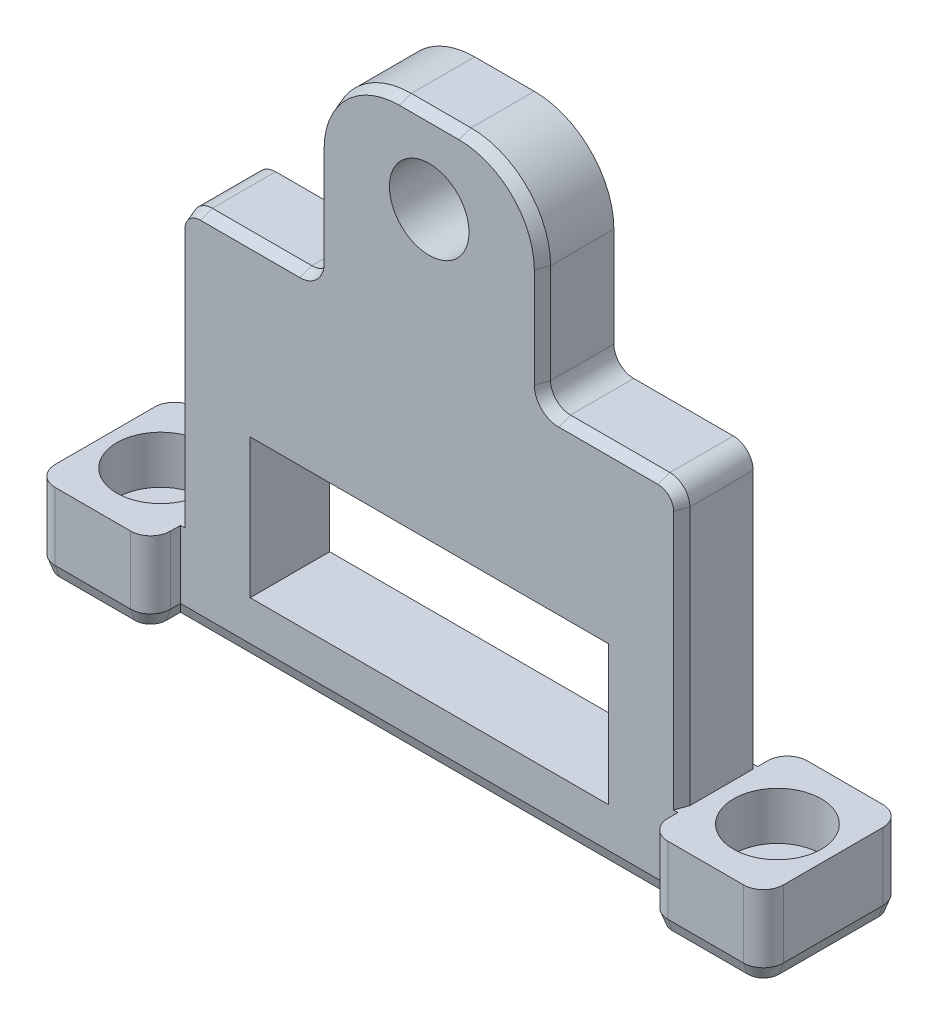
from build123d import *
from OCP.BRepFilletAPI import BRepFilletAPI_MakeChamfer

# Parameters (mm, degrees)
SKETCH1_W           = 12.5
SKETCH1_H           = 14
BOSS_EXTRUDE1_DEPTH = 2
SKETCH2_R           = 1
SKETCH2_W           = 9
SKETCH2_H           = 3.5
SKETCH2_W_2         = 3.5
SKETCH2_H_2         = 5
CUT_EXTRUDE1_DEPTH  = 3
FILLET1_R           = 2
SKETCH4_W           = 2.9
SKETCH4_H           = 3.5
BOSS_EXTRUDE2_DEPTH = 2
SKETCH5_R           = 1.1
CUT_EXTRUDE3_DEPTH  = 1.2
FILLET2_R           = 0.5
FILLET3_R           = 0.5
CHAMFER1_SIZE       = 0.3
CHAMFER1_SIZE2      = 0.10919107


with BuildPart() as part:
    # Sketch1 → Boss-Extrude1 (new body)
    with BuildSketch(Plane.XY):
        Rectangle(SKETCH1_W, SKETCH1_H)
    extrude(amount=BOSS_EXTRUDE1_DEPTH)

    # Sketch2 → Cut-Extrude1 (cut)
    with BuildSketch(Plane.XY.offset(2)):
        with Locations((0, 5)):
            Circle(SKETCH2_R)
        with Locations((0, -3.95)):
            Rectangle(SKETCH2_W, SKETCH2_H)
        with Locations((-4.5, 4.5)):
            Rectangle(SKETCH2_W_2, SKETCH2_H_2)
        with Locations((4.5, 4.5)):
            Rectangle(SKETCH2_W_2, SKETCH2_H_2)
    extrude(amount=-CUT_EXTRUDE1_DEPTH, mode=Mode.SUBTRACT)

    # Fillet1
    fillet1_edges = [part.edges().sort_by_distance(p)[0] for p in [
        (-2.75, 7, 1),
        (2.75, 7, 1),
    ]]
    fillet(fillet1_edges, radius=FILLET1_R)

    # Sketch4 → Boss-Extrude2 (add)
    with BuildSketch(Plane.XZ.offset(7)):
        with Locations((-7.7, 1)):
            Rectangle(SKETCH4_W, SKETCH4_H)
        with Locations((7.7, 1)):
            Rectangle(SKETCH4_W, SKETCH4_H)
    extrude(amount=-BOSS_EXTRUDE2_DEPTH)

    # Sketch5 → Cut-Extrude3 (cut)
    with BuildSketch(Plane(origin=(0, -5, 0), x_dir=(1, 0, 0), z_dir=(0, 1, 0))):
        with Locations(Location((-7.75, -1, 0), (0, 0, 270))):
            Circle(SKETCH5_R)
        with Locations(Location((7.75, -1, 0), (0, 0, 270))):
            Circle(SKETCH5_R)
    extrude(amount=-CUT_EXTRUDE3_DEPTH, mode=Mode.SUBTRACT)

    # Fillet2
    fillet2_edges = [part.edges().sort_by_distance(p)[0] for p in [
        (6.25, -6, -0.75),
        (6.25, -6, 2.75),
        (9.15, -6, 2.75),
        (9.15, -6, -0.75),
        (-6.25, 2, 1),
        (6.25, 2, 1),
        (-6.25, -6, 2.75),
        (-6.25, -6, -0.75),
        (-9.15, -6, -0.75),
        (-9.15, -6, 2.75),
    ]]
    fillet(fillet2_edges, radius=FILLET2_R)

    # Fillet3
    fillet3_edges = [part.edges().sort_by_distance(p)[0] for p in [
        (-2.75, 2, 1),
        (2.75, 2, 1),
    ]]
    fillet(fillet3_edges, radius=FILLET3_R)

    # Chamfer1: one chamfer whose edges measure the first distance from different faces: ONE call of the kernel's chamfer builder (chamfer() names one face for all edges)
    chamfer1_edges_1 = [part.edges().sort_by_distance(p)[0] for p in [
        (-9.003553391, -7, -0.603553391),
    ]]
    chamfer1_side_1 = [part.faces().sort_by_distance(p)[0] for p in [
        (-9.003553391, -6, -0.603553391),
    ]]
    chamfer1_edges_2 = [part.edges().sort_by_distance(p)[0] for p in [
        (-9.15, -7, 1),
    ]]
    chamfer1_side_2 = [part.faces().sort_by_distance(p)[0] for p in [
        (-9.15, -6, 1),
    ]]
    chamfer1_edges_3 = [part.edges().sort_by_distance(p)[0] for p in [
        (-9.003553391, -7, 2.603553391),
    ]]
    chamfer1_side_3 = [part.faces().sort_by_distance(p)[0] for p in [
        (-9.003553391, -6, 2.603553391),
    ]]
    chamfer1_edges_4 = [part.edges().sort_by_distance(p)[0] for p in [
        (-7.7, -7, 2.75),
    ]]
    chamfer1_side_4 = [part.faces().sort_by_distance(p)[0] for p in [
        (-7.7, -6, 2.75),
    ]]
    chamfer1_edges_5 = [part.edges().sort_by_distance(p)[0] for p in [
        (-6.396446609, -7, 2.603553391),
    ]]
    chamfer1_side_5 = [part.faces().sort_by_distance(p)[0] for p in [
        (-6.396446609, -6, 2.603553391),
    ]]
    chamfer1_edges_6 = [part.edges().sort_by_distance(p)[0] for p in [
        (-6.25, -7, 2.125),
    ]]
    chamfer1_side_6 = [part.faces().sort_by_distance(p)[0] for p in [
        (-6.25, -6, 2.125),
    ]]
    chamfer1_edges_7 = [part.edges().sort_by_distance(p)[0] for p in [
        (0, -7, 2),
    ]]
    chamfer1_side_7 = [part.faces().sort_by_distance(p)[0] for p in [
        (0, -0.579012096, 2),
    ]]
    chamfer1_edges_8 = [part.edges().sort_by_distance(p)[0] for p in [
        (6.25, -7, 2.125),
    ]]
    chamfer1_side_8 = [part.faces().sort_by_distance(p)[0] for p in [
        (6.25, -6, 2.125),
    ]]
    chamfer1_edges_9 = [part.edges().sort_by_distance(p)[0] for p in [
        (6.396446609, -7, 2.603553391),
    ]]
    chamfer1_side_9 = [part.faces().sort_by_distance(p)[0] for p in [
        (6.396446609, -6, 2.603553391),
    ]]
    chamfer1_edges_10 = [part.edges().sort_by_distance(p)[0] for p in [
        (7.7, -7, 2.75),
    ]]
    chamfer1_side_10 = [part.faces().sort_by_distance(p)[0] for p in [
        (7.7, -6, 2.75),
    ]]
    chamfer1_edges_11 = [part.edges().sort_by_distance(p)[0] for p in [
        (9.003553391, -7, 2.603553391),
    ]]
    chamfer1_side_11 = [part.faces().sort_by_distance(p)[0] for p in [
        (9.003553391, -6, 2.603553391),
    ]]
    chamfer1_edges_12 = [part.edges().sort_by_distance(p)[0] for p in [
        (9.15, -7, 1),
    ]]
    chamfer1_side_12 = [part.faces().sort_by_distance(p)[0] for p in [
        (9.15, -6, 1),
    ]]
    chamfer1_edges_13 = [part.edges().sort_by_distance(p)[0] for p in [
        (9.003553391, -7, -0.603553391),
    ]]
    chamfer1_side_13 = [part.faces().sort_by_distance(p)[0] for p in [
        (9.003553391, -6, -0.603553391),
    ]]
    chamfer1_edges_14 = [part.edges().sort_by_distance(p)[0] for p in [
        (7.7, -7, -0.75),
    ]]
    chamfer1_side_14 = [part.faces().sort_by_distance(p)[0] for p in [
        (7.7, -6, -0.75),
    ]]
    chamfer1_edges_15 = [part.edges().sort_by_distance(p)[0] for p in [
        (6.396446609, -7, -0.603553391),
    ]]
    chamfer1_side_15 = [part.faces().sort_by_distance(p)[0] for p in [
        (6.396446609, -6, -0.603553391),
    ]]
    chamfer1_edges_16 = [part.edges().sort_by_distance(p)[0] for p in [
        (6.25, -7, -0.125),
    ]]
    chamfer1_side_16 = [part.faces().sort_by_distance(p)[0] for p in [
        (6.25, -6, -0.125),
    ]]
    chamfer1_edges_17 = [part.edges().sort_by_distance(p)[0] for p in [
        (0, -7, 0),
        (6.25, -1.75, 0),
        (6.103553391, 1.853553391, 0),
        (2.896446609, 2.146446609, 0),
        (2.75, 3.75, 0),
        (2.164213562, 6.414213562, 0),
        (0, 7, 0),
        (-2.164213562, 6.414213562, 0),
        (-2.75, 3.75, 0),
        (-2.896446609, 2.146446609, 0),
        (-6.103553391, 1.853553391, 0),
        (-6.25, -1.75, 0),
        (4.5, 2, 0),
        (-4.5, 2, 0),
    ]]
    chamfer1_side_17 = [part.faces().sort_by_distance(p)[0] for p in [
        (0, -0.579012096, 0),
    ]]
    chamfer1_edges_18 = [part.edges().sort_by_distance(p)[0] for p in [
        (-6.25, -7, -0.125),
    ]]
    chamfer1_side_18 = [part.faces().sort_by_distance(p)[0] for p in [
        (-6.25, -6, -0.125),
    ]]
    chamfer1_edges_19 = [part.edges().sort_by_distance(p)[0] for p in [
        (-6.396446609, -7, -0.603553391),
    ]]
    chamfer1_side_19 = [part.faces().sort_by_distance(p)[0] for p in [
        (-6.396446609, -6, -0.603553391),
    ]]
    chamfer1_edges_20 = [part.edges().sort_by_distance(p)[0] for p in [
        (-7.7, -7, -0.75),
    ]]
    chamfer1_side_20 = [part.faces().sort_by_distance(p)[0] for p in [
        (-7.7, -6, -0.75),
    ]]
    chamfer1_edges_21 = [part.edges().sort_by_distance(p)[0] for p in [
        (6.25, -1.75, 2),
    ]]
    chamfer1_side_21 = [part.faces().sort_by_distance(p)[0] for p in [
        (6.25, -1.75, 1),
    ]]
    chamfer1_edges_22 = [part.edges().sort_by_distance(p)[0] for p in [
        (6.103553391, 1.853553391, 2),
    ]]
    chamfer1_side_22 = [part.faces().sort_by_distance(p)[0] for p in [
        (6.103553391, 1.853553391, 1),
    ]]
    chamfer1_edges_23 = [part.edges().sort_by_distance(p)[0] for p in [
        (2.896446609, 2.146446609, 2),
    ]]
    chamfer1_side_23 = [part.faces().sort_by_distance(p)[0] for p in [
        (2.896446609, 2.146446609, 1),
    ]]
    chamfer1_edges_24 = [part.edges().sort_by_distance(p)[0] for p in [
        (2.75, 3.75, 2),
    ]]
    chamfer1_side_24 = [part.faces().sort_by_distance(p)[0] for p in [
        (2.75, 3.75, 1),
    ]]
    chamfer1_edges_25 = [part.edges().sort_by_distance(p)[0] for p in [
        (2.164213562, 6.414213562, 2),
    ]]
    chamfer1_side_25 = [part.faces().sort_by_distance(p)[0] for p in [
        (2.164213562, 6.414213562, 1),
    ]]
    chamfer1_edges_26 = [part.edges().sort_by_distance(p)[0] for p in [
        (0, 7, 2),
    ]]
    chamfer1_side_26 = [part.faces().sort_by_distance(p)[0] for p in [
        (0, 7, 1),
    ]]
    chamfer1_edges_27 = [part.edges().sort_by_distance(p)[0] for p in [
        (-2.164213562, 6.414213562, 2),
    ]]
    chamfer1_side_27 = [part.faces().sort_by_distance(p)[0] for p in [
        (-2.164213562, 6.414213562, 1),
    ]]
    chamfer1_edges_28 = [part.edges().sort_by_distance(p)[0] for p in [
        (-2.75, 3.75, 2),
    ]]
    chamfer1_side_28 = [part.faces().sort_by_distance(p)[0] for p in [
        (-2.75, 3.75, 1),
    ]]
    chamfer1_edges_29 = [part.edges().sort_by_distance(p)[0] for p in [
        (-2.896446609, 2.146446609, 2),
    ]]
    chamfer1_side_29 = [part.faces().sort_by_distance(p)[0] for p in [
        (-2.896446609, 2.146446609, 1),
    ]]
    chamfer1_edges_30 = [part.edges().sort_by_distance(p)[0] for p in [
        (-6.103553391, 1.853553391, 2),
    ]]
    chamfer1_side_30 = [part.faces().sort_by_distance(p)[0] for p in [
        (-6.103553391, 1.853553391, 1),
    ]]
    chamfer1_edges_31 = [part.edges().sort_by_distance(p)[0] for p in [
        (-6.25, -1.75, 2),
    ]]
    chamfer1_side_31 = [part.faces().sort_by_distance(p)[0] for p in [
        (-6.25, -1.75, 1),
    ]]
    chamfer1_edges_32 = [part.edges().sort_by_distance(p)[0] for p in [
        (4.5, 2, 2),
    ]]
    chamfer1_side_32 = [part.faces().sort_by_distance(p)[0] for p in [
        (4.5, 2, 1),
    ]]
    chamfer1_edges_33 = [part.edges().sort_by_distance(p)[0] for p in [
        (-4.5, 2, 2),
    ]]
    chamfer1_side_33 = [part.faces().sort_by_distance(p)[0] for p in [
        (-4.5, 2, 1),
    ]]
    chamfer1 = BRepFilletAPI_MakeChamfer(part.part.solid().wrapped)
    for e in chamfer1_edges_1:
        chamfer1.Add(CHAMFER1_SIZE, CHAMFER1_SIZE2, e.wrapped, chamfer1_side_1[0].wrapped)  # the first distance lies on this face
    for e in chamfer1_edges_2:
        chamfer1.Add(CHAMFER1_SIZE, CHAMFER1_SIZE2, e.wrapped, chamfer1_side_2[0].wrapped)  # the first distance lies on this face
    for e in chamfer1_edges_3:
        chamfer1.Add(CHAMFER1_SIZE, CHAMFER1_SIZE2, e.wrapped, chamfer1_side_3[0].wrapped)  # the first distance lies on this face
    for e in chamfer1_edges_4:
        chamfer1.Add(CHAMFER1_SIZE, CHAMFER1_SIZE2, e.wrapped, chamfer1_side_4[0].wrapped)  # the first distance lies on this face
    for e in chamfer1_edges_5:
        chamfer1.Add(CHAMFER1_SIZE, CHAMFER1_SIZE2, e.wrapped, chamfer1_side_5[0].wrapped)  # the first distance lies on this face
    for e in chamfer1_edges_6:
        chamfer1.Add(CHAMFER1_SIZE, CHAMFER1_SIZE2, e.wrapped, chamfer1_side_6[0].wrapped)  # the first distance lies on this face
    for e in chamfer1_edges_7:
        chamfer1.Add(CHAMFER1_SIZE, CHAMFER1_SIZE2, e.wrapped, chamfer1_side_7[0].wrapped)  # the first distance lies on this face
    for e in chamfer1_edges_8:
        chamfer1.Add(CHAMFER1_SIZE, CHAMFER1_SIZE2, e.wrapped, chamfer1_side_8[0].wrapped)  # the first distance lies on this face
    for e in chamfer1_edges_9:
        chamfer1.Add(CHAMFER1_SIZE, CHAMFER1_SIZE2, e.wrapped, chamfer1_side_9[0].wrapped)  # the first distance lies on this face
    for e in chamfer1_edges_10:
        chamfer1.Add(CHAMFER1_SIZE, CHAMFER1_SIZE2, e.wrapped, chamfer1_side_10[0].wrapped)  # the first distance lies on this face
    for e in chamfer1_edges_11:
        chamfer1.Add(CHAMFER1_SIZE, CHAMFER1_SIZE2, e.wrapped, chamfer1_side_11[0].wrapped)  # the first distance lies on this face
    for e in chamfer1_edges_12:
        chamfer1.Add(CHAMFER1_SIZE, CHAMFER1_SIZE2, e.wrapped, chamfer1_side_12[0].wrapped)  # the first distance lies on this face
    for e in chamfer1_edges_13:
        chamfer1.Add(CHAMFER1_SIZE, CHAMFER1_SIZE2, e.wrapped, chamfer1_side_13[0].wrapped)  # the first distance lies on this face
    for e in chamfer1_edges_14:
        chamfer1.Add(CHAMFER1_SIZE, CHAMFER1_SIZE2, e.wrapped, chamfer1_side_14[0].wrapped)  # the first distance lies on this face
    for e in chamfer1_edges_15:
        chamfer1.Add(CHAMFER1_SIZE, CHAMFER1_SIZE2, e.wrapped, chamfer1_side_15[0].wrapped)  # the first distance lies on this face
    for e in chamfer1_edges_16:
        chamfer1.Add(CHAMFER1_SIZE, CHAMFER1_SIZE2, e.wrapped, chamfer1_side_16[0].wrapped)  # the first distance lies on this face
    for e in chamfer1_edges_17:
        chamfer1.Add(CHAMFER1_SIZE, CHAMFER1_SIZE2, e.wrapped, chamfer1_side_17[0].wrapped)  # the first distance lies on this face
    for e in chamfer1_edges_18:
        chamfer1.Add(CHAMFER1_SIZE, CHAMFER1_SIZE2, e.wrapped, chamfer1_side_18[0].wrapped)  # the first distance lies on this face
    for e in chamfer1_edges_19:
        chamfer1.Add(CHAMFER1_SIZE, CHAMFER1_SIZE2, e.wrapped, chamfer1_side_19[0].wrapped)  # the first distance lies on this face
    for e in chamfer1_edges_20:
        chamfer1.Add(CHAMFER1_SIZE, CHAMFER1_SIZE2, e.wrapped, chamfer1_side_20[0].wrapped)  # the first distance lies on this face
    for e in chamfer1_edges_21:
        chamfer1.Add(CHAMFER1_SIZE, CHAMFER1_SIZE2, e.wrapped, chamfer1_side_21[0].wrapped)  # the first distance lies on this face
    for e in chamfer1_edges_22:
        chamfer1.Add(CHAMFER1_SIZE, CHAMFER1_SIZE2, e.wrapped, chamfer1_side_22[0].wrapped)  # the first distance lies on this face
    for e in chamfer1_edges_23:
        chamfer1.Add(CHAMFER1_SIZE, CHAMFER1_SIZE2, e.wrapped, chamfer1_side_23[0].wrapped)  # the first distance lies on this face
    for e in chamfer1_edges_24:
        chamfer1.Add(CHAMFER1_SIZE, CHAMFER1_SIZE2, e.wrapped, chamfer1_side_24[0].wrapped)  # the first distance lies on this face
    for e in chamfer1_edges_25:
        chamfer1.Add(CHAMFER1_SIZE, CHAMFER1_SIZE2, e.wrapped, chamfer1_side_25[0].wrapped)  # the first distance lies on this face
    for e in chamfer1_edges_26:
        chamfer1.Add(CHAMFER1_SIZE, CHAMFER1_SIZE2, e.wrapped, chamfer1_side_26[0].wrapped)  # the first distance lies on this face
    for e in chamfer1_edges_27:
        chamfer1.Add(CHAMFER1_SIZE, CHAMFER1_SIZE2, e.wrapped, chamfer1_side_27[0].wrapped)  # the first distance lies on this face
    for e in chamfer1_edges_28:
        chamfer1.Add(CHAMFER1_SIZE, CHAMFER1_SIZE2, e.wrapped, chamfer1_side_28[0].wrapped)  # the first distance lies on this face
    for e in chamfer1_edges_29:
        chamfer1.Add(CHAMFER1_SIZE, CHAMFER1_SIZE2, e.wrapped, chamfer1_side_29[0].wrapped)  # the first distance lies on this face
    for e in chamfer1_edges_30:
        chamfer1.Add(CHAMFER1_SIZE, CHAMFER1_SIZE2, e.wrapped, chamfer1_side_30[0].wrapped)  # the first distance lies on this face
    for e in chamfer1_edges_31:
        chamfer1.Add(CHAMFER1_SIZE, CHAMFER1_SIZE2, e.wrapped, chamfer1_side_31[0].wrapped)  # the first distance lies on this face
    for e in chamfer1_edges_32:
        chamfer1.Add(CHAMFER1_SIZE, CHAMFER1_SIZE2, e.wrapped, chamfer1_side_32[0].wrapped)  # the first distance lies on this face
    for e in chamfer1_edges_33:
        chamfer1.Add(CHAMFER1_SIZE, CHAMFER1_SIZE2, e.wrapped, chamfer1_side_33[0].wrapped)  # the first distance lies on this face
    add(Compound.cast(chamfer1.Shape()), mode=Mode.REPLACE)


solid = part.part
